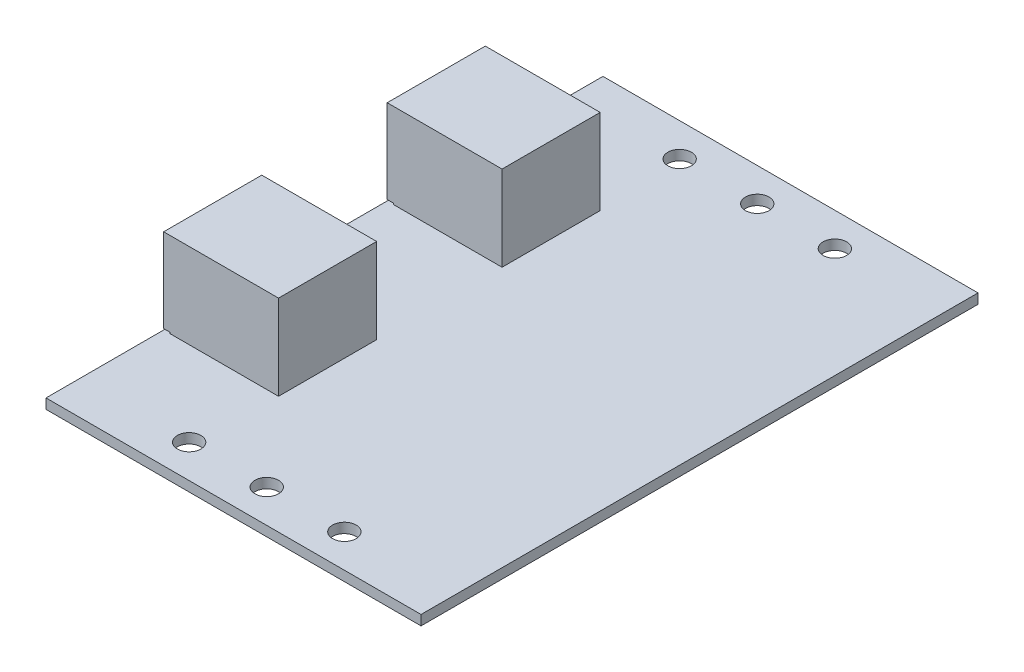
SolidWorks part; units mm, degrees
ref_plane "前视基准面" through (0, 0, 0) normal (0, 0, 1) x (1, 0, 0)
ref_plane "上视基准面" through (0, 0, 0) normal (0, 1, 0) x (1, 0, 0)
ref_plane "右视基准面" through (0, 0, 0) normal (1, 0, 0) x (0, 0, -1)
sketch "草图1" plane through (0, 0, 0) normal (0, 1, 0) x (1, 0, 0)
  line L1 (-30.2, 44.85) -> (30.2, 44.85)
  line L2 (-30.2, 44.85) -> (-30.2, -44.85)
  line L3 (-30.2, -44.85) -> (30.2, -44.85)
  line L4 (30.2, 44.85) -> (30.2, -44.85)
  line L5 (-30.2, 44.85) -> (30.2, -44.85) construction
  line L6 (-30.2, -44.85) -> (30.2, 44.85) construction
  point P0 (0, 0)
  dimension "D1" = 60.4
  dimension "D2" = 89.7
extrude "凸台-拉伸1" add sketch "草图1" along normal blind 1.6
sketch "草图2" plane through (0, 1.6, 0) normal (0, 1, 0) x (1, 0, 0)
  line L1 (-12.5, 39.5) -> (12.5, 39.5) construction
  line L2 (-12.5, 39.5) -> (-12.5, -39.5) construction
  line L3 (-12.5, -39.5) -> (12.5, -39.5) construction
  line L4 (12.5, 39.5) -> (12.5, -39.5) construction
  line L5 (-12.5, 39.5) -> (12.5, -39.5) construction
  line L6 (-12.5, -39.5) -> (12.5, 39.5) construction
  circle A0 centre (-12.5, -39.5) radius 1.9
  circle A1 centre (12.5, -39.5) radius 1.9
  circle A2 centre (-12.5, 39.5) radius 1.9
  circle A3 centre (12.5, 39.5) radius 1.9
  circle A4 centre (0, 39.5) radius 1.9
  circle A5 centre (0, -39.5) radius 1.9
  point P0 (0, 0)
  dimension "D1" = 3.8
  dimension "D2" = 25
  dimension "D3" = 79
extrude "切除-拉伸1" cut sketch "草图2" against normal blind 1.6
sketch "草图3" plane through (-30.2, 0, 0) normal (-1, 0, 0) x (0, 0, 1)
  line L0 (0, 0) -> (0, 13.8824) construction
  line L1 (10.1, 15.3) -> (25.9, 15.3)
  line L2 (10.1, 15.3) -> (10.1, 1.6)
  line L3 (10.1, 1.6) -> (25.9, 1.6)
  line L4 (25.9, 15.3) -> (25.9, 1.6)
  line L5 (-25.9, 15.3) -> (-10.1, 15.3)
  line L6 (-25.9, 15.3) -> (-25.9, 1.6)
  line L7 (-25.9, 1.6) -> (-10.1, 1.6)
  line L8 (-10.1, 15.3) -> (-10.1, 1.6)
  line L9 (-44.85, 1.6) -> (44.85, 1.6) construction
  line L10 (-44.85, 0) -> (44.85, 0) construction
  dimension "D1" = 15.8
  dimension "D2" = 15.3
  dimension "D3" = 36
extrude "凸台-拉伸2" add sketch "草图3" against normal blind 18.5
sketch "草图4" plane through (-30.2, 0, 0) normal (-1, 0, 0) x (0, 0, 1)
  line L0 (25.9, 1.6) -> (25.9, 15.3) construction
  line L1 (-25.9, 1.6) -> (25.9, 1.6)
  line L2 (-25.9, 1.6) -> (-25.9, 1.8)
  line L3 (-25.9, 1.8) -> (25.9, 1.8)
  line L4 (25.9, 1.6) -> (25.9, 1.8)
  dimension "D1" = 0.2
extrude "切除-拉伸2" cut sketch "草图4" against normal blind 1
sketch "草图5" plane through (-30.2, 0, 0) normal (-1, 0, 0) x (0, 0, 1)
  line L0 (-18, 15.3) -> (-18, 1.8) construction
  line L1 (-10.1, 15.3) -> (-25.9, 15.3) construction
  line L2 (-10.1, 1.8) -> (-25.9, 1.8) construction
  line L3 (18, 15.3) -> (18, 1.8) construction
  line L4 (25.9, 15.3) -> (10.1, 15.3) construction
  line L5 (25.9, 1.8) -> (10.1, 1.8) construction
  line L7 (11.6037, 13.8674) -> (24.3963, 13.8674)
  line L8 (11.6037, 13.8674) -> (11.6037, 3.2326)
  line L9 (11.6037, 3.2326) -> (24.3963, 3.2326)
  line L10 (24.3963, 13.8674) -> (24.3963, 3.2326)
  line L11 (11.6037, 13.8674) -> (24.3963, 3.2326) construction
  line L12 (11.6037, 3.2326) -> (24.3963, 13.8674) construction
  line L13 (-24.4974, 14.18) -> (-11.5026, 14.18)
  line L14 (-24.4974, 14.18) -> (-24.4974, 2.92)
  line L15 (-24.4974, 2.92) -> (-11.5026, 2.92)
  line L16 (-11.5026, 14.18) -> (-11.5026, 2.92)
  line L17 (-24.4974, 14.18) -> (-11.5026, 2.92) construction
  line L18 (-24.4974, 2.92) -> (-11.5026, 14.18) construction
  point P12 (18, 8.55)
  point P17 (-18, 8.55)
extrude "切除-拉伸3" cut sketch "草图5" against normal blind 1
